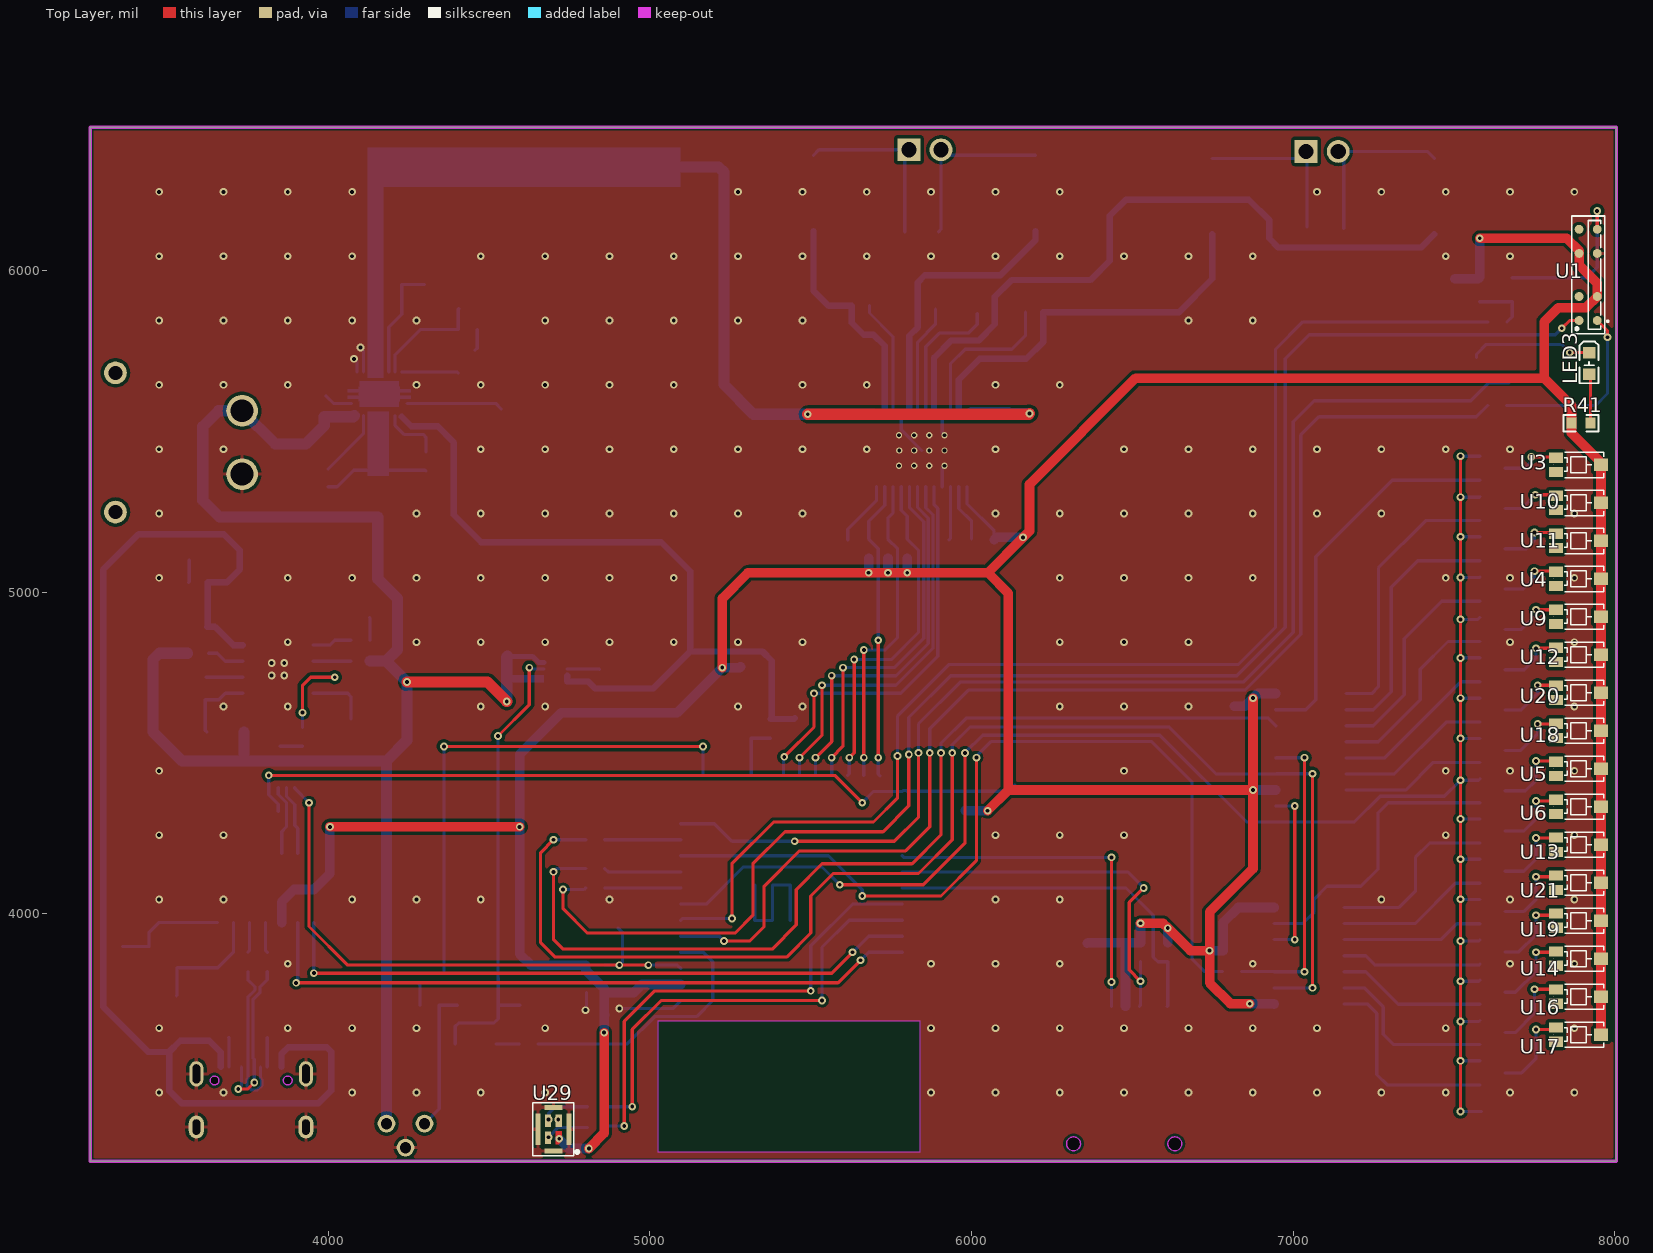
[diagram p0: Top Layer view]
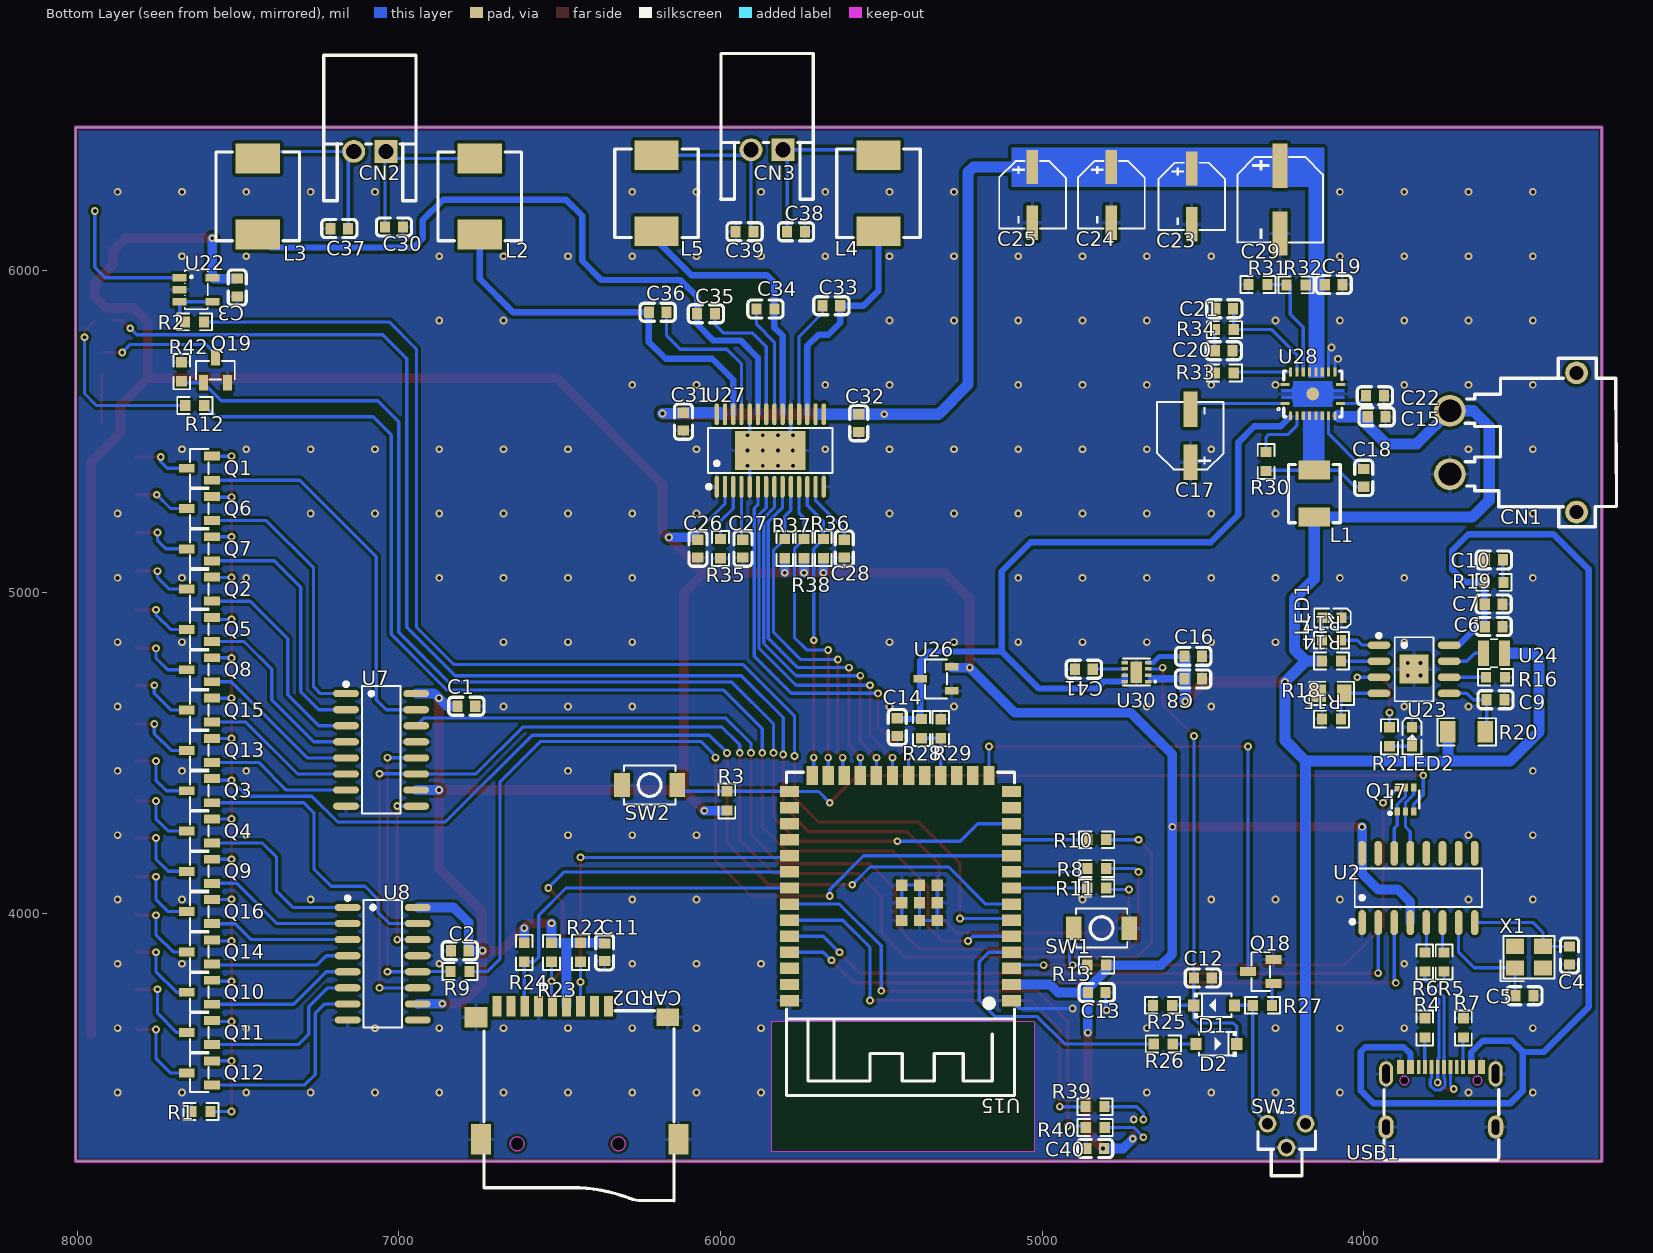
[diagram p1: Bottom Layer view, seen from below]
# Altium PCB MISC75432.pcbdoc (part 1 of 2)
Units mil, origin at the board's own origin, x right, y up, seen from the top; angles counter-clockwise.
Board outline 4745 x 3215 mil, 2 copper layers (Top Layer, Bottom Layer), stack 62.206 mil thick; 150 components, 141 nets, 533 pads, 333 vias.

## Layer stack, top to bottom
Top Solder Mask Layer: solder mask 0.394, Dk 3.3
Top Layer: signal copper 1.379
Dielectric1: surface 59.449, FR4, Dk 4.5
Bottom Layer: signal copper 1.378
Bottom Solder Mask Layer: solder mask 0.394, Dk 3.3

## Board outline
3260,6445 3260,3230 8005,3230 8005,6445

## Design rules (kind name [scope] priority, off if disabled: settings)
BoardOutlineClearance copperThickness2oz_1 [All] p2: genericclearance=7.99 ignorepadtopadclearanceinfootprint=FALSE except(0: Arc-SplitContinuation Track-SplitContinuation SMDPad-SplitContinuation THPad-SplitContinuation Via-SplitContinuation Fill-SplitContinuation Region-SplitContinuation Poly-SplitContinuation Text-SplitContinuation Hole-SplitContinuation; 5.98: Arc-CutoutEdge SMDPad-CutoutEdge THPad-CutoutEdge Via-CutoutEdge Fill-CutoutEdge Region-CutoutEdge Text-CutoutEdge; 6.93: Hole-OutlineEdge Hole-CutoutEdge; 10: Poly-OutlineEdge Poly-CutoutEdge; 11.81: Arc-OutlineEdge Track-OutlineEdge SMDPad-OutlineEdge THPad-OutlineEdge Via-OutlineEdge Fill-OutlineEdge Region-OutlineEdge Text-OutlineEdge Track-CutoutEdge)
BoardOutlineClearance copperThickness1oz_1 [All] p4: genericclearance=4.02 ignorepadtopadclearanceinfootprint=FALSE except(0: Arc-SplitContinuation Track-SplitContinuation SMDPad-SplitContinuation THPad-SplitContinuation Via-SplitContinuation Fill-SplitContinuation Region-SplitContinuation Poly-SplitContinuation Text-SplitContinuation Hole-SplitContinuation; 5.98: SMDPad-CutoutEdge THPad-CutoutEdge Via-CutoutEdge Fill-CutoutEdge Region-CutoutEdge Text-CutoutEdge; 6.93: Hole-OutlineEdge Hole-CutoutEdge; 10: Poly-OutlineEdge Poly-CutoutEdge; 11.81: Arc-OutlineEdge Track-OutlineEdge SMDPad-OutlineEdge THPad-OutlineEdge Via-OutlineEdge Fill-OutlineEdge Region-OutlineEdge Text-OutlineEdge Arc-CutoutEdge Track-CutoutEdge)
Clearance copperThickness2oz [(InNet('OUT_A-') OR InNet('OUT_A+') OR InNet('OUT_B-') OR InNet('OUT_B+'))] p1: gap=7.99 ignorepadtopadclearanceinfootprint=FALSE except(5.98: SMDPad-Track SMDPad-SMDPad THPad-Track SMDPad-THPad THPad-THPad Track-Via SMDPad-Via THPad-Via Via-Via Fill-Track Region-Track Fill-SMDPad Region-SMDPad Fill-THPad Region-THPad Fill-Via Region-Via Fill-Fill Fill-Region Region-Region Arc-Track Arc-SMDPad Arc-THPad Arc-Via Fill-Arc Region-Arc Arc-Arc Text-Track SMDPad-Text Text-THPad Text-Via Fill-Text Region-Text Arc-Text Text-Text; 6.93: Hole-Track Hole-SMDPad Hole-THPad Hole-Via Fill-Hole Region-Hole Hole-Arc Hole-Text; 10: Poly-Track Poly-SMDPad Poly-THPad Poly-Via Poly-Fill Poly-Region Poly-Poly Poly-Arc Poly-Text Poly-Hole)
Clearance copperThickness1oz [All] p3: gap=4.02 ignorepadtopadclearanceinfootprint=FALSE except(5.98: SMDPad-Track SMDPad-SMDPad THPad-Track SMDPad-THPad THPad-THPad Track-Via SMDPad-Via THPad-Via Via-Via Fill-Track Region-Track Fill-SMDPad Region-SMDPad Fill-THPad Region-THPad Fill-Via Region-Via Fill-Fill Fill-Region Region-Region Arc-Track Arc-SMDPad Arc-THPad Arc-Via Fill-Arc Region-Arc Arc-Arc Text-Track SMDPad-Text Text-THPad Text-Via Fill-Text Region-Text Arc-Text Text-Text; 6.93: Hole-Track Hole-SMDPad Hole-THPad Hole-Via Fill-Hole Region-Hole Hole-Arc Hole-Text; 10: Poly-Track Poly-SMDPad Poly-THPad Poly-Via Poly-Fill Poly-Region Poly-Poly Poly-Arc Poly-Text Poly-Hole)
DiffPairsRouting differentialPair [All] p1: maxlimit=6 minlimit=6 mostfreqgap=6 toplayer_minwidth=5 toplayer_prefwidth=10 toplayer_maxwidth=100 toplayer_mingap=6 toplayer_prefgap=6 toplayer_maxgap=6 bottomlayer_minwidth=5 bottomlayer_prefwidth=10 bottomlayer_maxwidth=100 bottomlayer_mingap=6 bottomlayer_prefgap=6 bottomlayer_maxgap=6 maxuncoupledlength=10
HoleToHoleClearance otherClearance [All] p1: gap=11.81 allowstackedmicrovias=TRUE
Length netLength [All] p1: minlimit=0 maxlimit=0
MatchedLengths netLengthTolerance [All] p1: tolerance=1000
PasteMaskExpansion pasteMaskExpansion [All] p1: expansion=0
PlaneConnect innerPlane [All] p1: planeconnectstyle=Relief reliefexpansion=20 reliefentries=4 reliefconductorwidth=10 reliefairgap=10
PolygonConnect copperRegion [(InNet('PD_GATE_15') OR InNet('IO0'))] p1: connectstyle=Relief reliefconductorwidth=10 reliefentries=4 polygonreliefangle="90 Angle" airgapwidth=10 via.connectstyle=Relief via.reliefconductorwidth=10 via.reliefentries=4 via.polygonreliefangle="90 Angle" via.airgapwidth=10
RoutingVias viaSize [All] p1: holewidth=12.01 width=24.02 viastyle="Through Hole" minholewidth=11.81 minwidth=19.68 maxholewidth=248.03 maxwidth=393.7
SolderMaskExpansion solderMaskExpansion [IsVia] p1: expansion=-1000 istentingtop=TRUE
SolderMaskExpansion solderMaskExpansion [All] p2: expansion=2 istentingtop=FALSE
Width copperThickness1oz_2 [All] p1 off: maxlimit=10 minlimit=10 preferedwidth=10 toplayer_minwidth=5 toplayer_maxwidth=100 toplayer_prefwidth=10 bottomlayer_minwidth=5 bottomlayer_maxwidth=100 bottomlayer_prefwidth=10
Width power_trackWidth1 [All] p2 off: maxlimit=10 minlimit=10 preferedwidth=10 toplayer_minwidth=23.6 toplayer_maxwidth=78.7 toplayer_prefwidth=39.4 bottomlayer_minwidth=23.6 bottomlayer_maxwidth=78.7 bottomlayer_prefwidth=39.4
Width trackWidth2 [(InNet('+12V') OR InNet('OUT_A-') OR InNet('OUT_A+') OR InNet('OUT_B-') OR InNet('OUT_B+') OR InNet('VBUS') OR InNet('VSYS_MAIN'))] p3: maxlimit=10 minlimit=10 preferedwidth=10 toplayer_minwidth=15.7 toplayer_maxwidth=39.4 toplayer_prefwidth=19.7 bottomlayer_minwidth=15.7 bottomlayer_maxwidth=39.4 bottomlayer_prefwidth=19.7
Width trackWidth3_BAT [(InNet('VBAT'))] p4: maxlimit=10 minlimit=10 preferedwidth=10 toplayer_minwidth=15.7 toplayer_maxwidth=100 toplayer_prefwidth=59.1 bottomlayer_minwidth=15.7 bottomlayer_maxwidth=100 bottomlayer_prefwidth=59.1
Width copperThickness2oz_2 [All] p5: maxlimit=10 minlimit=10 preferedwidth=10 toplayer_minwidth=8 toplayer_maxwidth=100 toplayer_prefwidth=10 bottomlayer_minwidth=8 bottomlayer_maxwidth=100 bottomlayer_prefwidth=10

## Components (designator, comment, footprint, x,y, rotation, side; value= is the part's Value field where it differs from the comment)
C1 "100nF" C0603 6790,4645 r180 bottom
C2 "100nF" C0603 6810,3885 r0 bottom
C3 "100nF" C0603 7502.44,5946.77 r270 bottom
C4 "22pF" C0603 3360,3870 r90 bottom
C5 "22pF" C0603 3500.12,3745 r0 bottom
C6 "10uF" C0603 3596.03,4892.5 r180 bottom
C7 "22uF" C0603 3596.03,4962.5 r180 bottom
C8 "22uF" C0603 4530,4730 r0 bottom
C9 "22uF" C0603 3590.12,4665 r0 bottom
C10 "10uF" C0603 3595,5100 r0 bottom
C11 "100nF" C0603 6360,3880 r90 bottom
C12 "100nF" C0603 4500,3800 r180 bottom
C13 "1uF" C0603 4830,3755 r0 bottom
C14 "1uF" C0603 5450,4580 r90 bottom
C15 "10uF" C0603 3960,5545 r180 bottom
C16 "100nF" C0603 4529.88,4800 r180 bottom
C17 "2.2uF" CAP-SMD_BD5.0-L5.3-W5.3-LS6.0-FD 4538.41,5485.99 r90 bottom
C18 "100nF" C0603 4000,5355 r270 bottom
C19 "1uF" C0603 4093.41,5955.99 r180 bottom
C20 "22uF" C0603 4435,5750 r180 bottom
C21 "33pF" C0603 4433.41,5880.99 r0 bottom
C22 "47nF" C0603 3965,5610 r180 bottom
C23 "22uF" CAP-SMD_BD5.0-L5.3-W5.3-LS6.3-FD-1 4535,6230 r270 bottom
C24 "22uF" CAP-SMD_BD5.0-L5.3-W5.3-LS6.3-FD-1 4785,6235 r270 bottom
C25 "22uF" CAP-SMD_BD5.0-L5.3-W5.3-LS6.3-FD-1 5030,6235 r270 bottom
C26 "100nF" C0603 6070,5135 r270 bottom
C27 "1uF" C0603 5930,5135 r270 bottom
C28 "1uF" C0603 5615,5135 r90 bottom
C29 "220uF" CAP-SMD_BD6.3-L6.6-W6.6-LS7.3-FD-H7.7 4260,6220 r270 bottom
C30 "680nF" C0603 7015,6135 r180 bottom
C31 "10uF" C0603 6115,5530 r90 bottom
C32 "100nF" C0603 5570,5525 r90 bottom
C33 "220nF" C0603 5655,5890 r180 bottom
C34 "220nF" C0603 5860,5880 r180 bottom
C35 "220nF" C0603 6045,5865 r0 bottom
C36 "220nF" C0603 6195,5870 r0 bottom
C37 "680nF" C0603 7185,6130 r180 bottom
C38 "680nF" C0603 5765,6120 r180 bottom
C39 "680nF" C0603 5925,6120 r180 bottom
C40 "100nF" C0603 4834.88,3270 r0 bottom
C41 "1nF" C0603 4870,4760 r0 bottom
CARD2 "TF-15x15" TF-SMD_TF-15-15 6445,3505 r270 bottom
CN1 "XT30PW-M30.G.Y" CONN-TH_XT30PW-M 3535,5465 r90 bottom
CN2 "S2B-XH-A-1(LF)(SN)" CONN-TH_S2B-XH-A-1-LF-SN 7090,6370 r180 bottom
CN3 "S2B-XH-A-1(LF)(SN)" CONN-TH_S2B-XH-A-1-LF-SN 5855,6375 r180 bottom
D1 "1N4148W" SOD-123_L2.7-W1.6-LS3.7-FD 4465,3715 r0 bottom
D2 "1N4148W" SOD-123_L2.7-W1.6-LS3.7-FD 4458.18,3595.01 r180 bottom
L1 "2.2uH" IND-SMD_L4.6-W4.1_MHCI04015 4153.41,5305.99 r270 bottom
L2 "10uH" IND-SMD_L7.3-W6.8 6748.6,6230 r90 bottom
L3 "10uH" IND-SMD_L7.3-W6.8 7438.6,6230 r90 bottom
L4 "10uH" IND-SMD_L7.3-W6.8 5508.6,6240 r90 bottom
L5 "10uH" IND-SMD_L7.3-W6.8 6198.6,6240 r90 bottom
LED1 "NCD0603Y2" LED0603-RD 4098.98,4919.99 r0 bottom
LED2 "NCD0603Y2" LED0603-RD 3850,4550 r270 bottom
LED3 "GL0603UR01" LED0603-FD 7920,5710 r90 top
Q1 "2N7002" SOT-23-3_L2.9-W1.3-P1.90-LS2.4-BR 7620,5385 r180 bottom
Q2 "2N7002" SOT-23-3_L2.9-W1.3-P1.90-LS2.4-BR 7620,5009 r180 bottom
Q3 "2N7002" SOT-23-3_L2.9-W1.3-P1.90-LS2.4-BR 7620,4382.33 r180 bottom
Q4 "2N7002" SOT-23-3_L2.9-W1.3-P1.90-LS2.4-BR 7620,4257 r180 bottom
Q5 "2N7002" SOT-23-3_L2.9-W1.3-P1.90-LS2.4-BR 7620,4883.67 r180 bottom
Q6 "2N7002" SOT-23-3_L2.9-W1.3-P1.90-LS2.4-BR 7620,5259.67 r180 bottom
Q7 "2N7002" SOT-23-3_L2.9-W1.3-P1.90-LS2.4-BR 7620,5134.33 r180 bottom
Q8 "2N7002" SOT-23-3_L2.9-W1.3-P1.90-LS2.4-BR 7620,4758.33 r180 bottom
Q9 "2N7002" SOT-23-3_L2.9-W1.3-P1.90-LS2.4-BR 7620,4131.67 r180 bottom
Q10 "2N7002" SOT-23-3_L2.9-W1.3-P1.90-LS2.4-BR 7620,3755.67 r180 bottom
Q11 "2N7002" SOT-23-3_L2.9-W1.3-P1.90-LS2.4-BR 7620,3630.33 r180 bottom
Q12 "2N7002" SOT-23-3_L2.9-W1.3-P1.90-LS2.4-BR 7620,3505 r180 bottom
Q13 "2N7002" SOT-23-3_L2.9-W1.3-P1.90-LS2.4-BR 7620,4507.67 r180 bottom
Q14 "2N7002" SOT-23-3_L2.9-W1.3-P1.90-LS2.4-BR 7620,3881 r180 bottom
Q15 "2N7002" SOT-23-3_L2.9-W1.3-P1.90-LS2.4-BR 7620,4633 r180 bottom
Q16 "2N7002" SOT-23-3_L2.9-W1.3-P1.90-LS2.4-BR 7620,4006.33 r180 bottom
Q17 "UMH3N" SC-70-6_L2.2-W1.3-P0.65-LS2.1-BR 3870,4355 r270 bottom
Q18 "2N7002" SOT-23-3_L2.9-W1.3-P1.90-LS2.4-BR 4320,3820 r180 bottom
Q19 "2N7002" SOT-23-3_L2.9-W1.3-P1.90-LS2.4-BR 7570,5690 r270 bottom
R1 "10kΩ" R0603 7615,3385 r0 bottom
R2 "49.9Ω" R0603 7635,5840 r180 bottom
R3 "10kΩ" R0603 5980,4350.68 r270 bottom
R4 "5.1kΩ" R0603 3810,3645 r270 bottom
R5 "27Ω" R0603 3750,3850 r270 bottom
R6 "27Ω" R0603 3810,3850 r270 bottom
R7 "5.1kΩ" R0603 3690,3645 r270 bottom
R8 "49.9Ω" R0603 4830,4140 r180 bottom
R9 "49.9Ω" R0603 6810,3820 r0 bottom
R10 "49.9Ω" R0603 4830,4230 r0 bottom
R11 "49.9Ω" R0603 4830,4080 r0 bottom
R12 "49.9Ω" R0603 7634.32,5580 r180 bottom
R13 "10kΩ" R0603 4830,3840 r0 bottom
R14 "1kΩ" R0603 4100,4785.34 r180 bottom
R15 "82kΩ" R0603 4100,4605 r180 bottom
R16 "47kΩ" R0603 3590,4735 r180 bottom
R17 "100Ω" R0603 4100,4850 r180 bottom
R18 "HNTC0805-104F3950FB" R0805 4100,4685 r180 bottom
R19 "2Ω" R0603 3595,5030 r180 bottom
R20 "500mΩ" R1206 3680,4565 r0 bottom
R21 "100Ω" R0603 3920,4550 r90 bottom
R22 "4.7kΩ" R0603 6435,3880 r270 bottom
R23 "4.7kΩ" R0603 6525,3880 r270 bottom
R24 "4.7kΩ" R0603 6610,3880 r270 bottom
R25 "1MΩ" R0603 4625,3715 r0 bottom
R26 "10kΩ" R0603 4623.18,3595.01 r180 bottom
R27 "100kΩ" R0603 4315,3715 r0 bottom
R28 "499kΩ" R0603 5374.66,4575.34 r90 bottom
R29 "100kΩ" R0603 5315,4575 r270 bottom
R30 "249kΩ" R0603 4303.41,5405.99 r270 bottom
R31 "20kΩ" R0603 4328.41,5955.99 r180 bottom
R32 "180kΩ" R0603 4210,5955 r180 bottom
R33 "100kΩ" R0603 4433.41,5680.99 r180 bottom
R34 "10kΩ" R0603 4433.41,5815.99 r0 bottom
R35 "4.7kΩ" R0603 6000,5135 r90 bottom
R36 "10kΩ" R0603 5680,5135 r90 bottom
R37 "2.2kΩ" R0603 5800,5135 r90 bottom
R38 "2.2kΩ" R0603 5740,5135 r90 bottom
R39 "33Ω" R0603 4835.68,3400 r180 bottom
R40 "33Ω" R0603 4834.66,3335.34 r180 bottom
R41 "56Ω" R0603 7895,5525 r0 top
R42 "10kΩ" R0603 7675,5685 r90 bottom
SW1 "TS-1088-AR02016" SW-SMD_L3.9-W3.0-P4.45 4815,3955 r0 bottom
SW2 "TS-1088-AR02016" SW-SMD_L3.9-W3.0-P4.45 6220,4400 r0 bottom
SW3 "TS-1009B-05026" SW-TH_3P-L4.5-W3.8-P3.10-LS1.9_TS-1009B-05026 4240,3310 r180 bottom
U1 "S13131-1536" BGA-8_L9.1-W2.4_S13131-1536 7917.16,5985.9 r90 top
U2 "CH340G" SOIC-16_L9.9-W3.9-P1.27-LS6.0-BL 3830,4080 r180 bottom
U3 "TEMT6000X01" SENSORS-SMD_TEMT6000X01 7886.89,5395.35 r0 top
U4 "TEMT6000X01" SENSORS-SMD_TEMT6000X01 7886.89,5041.02 r0 top
U5 "TEMT6000X01" SENSORS-SMD_TEMT6000X01 7886.89,4450.47 r0 top
U6 "TEMT6000X01" SENSORS-SMD_TEMT6000X01 7886.89,4332.36 r0 top
U7 "74HC595" SOP-16_L9.9-W3.9-P1.27-LS6.0-BL 7055,4509.33 r270 bottom
U8 "74HC595" SOP-16_L9.9-W3.9-P1.27-LS6.0-BL 7050,3844.33 r270 bottom
U9 "TEMT6000X01" SENSORS-SMD_TEMT6000X01 7886.89,4922.91 r0 top
U10 "TEMT6000X01" SENSORS-SMD_TEMT6000X01 7886.89,5277.24 r0 top
U11 "TEMT6000X01" SENSORS-SMD_TEMT6000X01 7886.89,5159.13 r0 top
U12 "TEMT6000X01" SENSORS-SMD_TEMT6000X01 7886.89,4804.8 r0 top
U13 "TEMT6000X01" SENSORS-SMD_TEMT6000X01 7886.89,4214.25 r0 top
U14 "TEMT6000X01" SENSORS-SMD_TEMT6000X01 7886.89,3859.92 r0 top
U15 "ESP32-S3-WROOM-1-N8R8" WIRELM-SMD_ESP32-S3-WROOM-1 5440,4080 r0 bottom
U16 "TEMT6000X01" SENSORS-SMD_TEMT6000X01 7886.89,3741.81 r0 top
U17 "TEMT6000X01" SENSORS-SMD_TEMT6000X01 7886.89,3623.7 r0 top
U18 "TEMT6000X01" SENSORS-SMD_TEMT6000X01 7886.89,4568.58 r0 top
U19 "TEMT6000X01" SENSORS-SMD_TEMT6000X01 7886.89,3978.03 r0 top
U20 "TEMT6000X01" SENSORS-SMD_TEMT6000X01 7886.89,4686.69 r0 top
U21 "TEMT6000X01" SENSORS-SMD_TEMT6000X01 7886.89,4096.14 r0 top
U22 "LMV321IDBVR" SOT-23-5_L3.0-W1.7-P0.95-LS2.8-BR 7630,5940 r0 bottom
U23 "IP2312U_VSET" SOP-8_L4.9-W3.9-P1.27-LS6.0-BL-EP 3843.52,4760 r270 bottom
U24 "1uH" IND-SMD_L2.5-W2.0-VLS252012CX-150M 3595,4810 r180 bottom
U26 "ME6211A33M3G-N" SOT-23-3_L2.9-W1.6-P1.90-LS2.8-BR 5330,4730 r180 bottom
U27 "TAS5805MPWPR" HTSSOP-28_L9.7-W4.4-P0.65-LS6.4-BL-EP 5845,5440 r180 bottom
U28 "TPS61088RHLR" VQFN-20_L4.6-W3.6-P0.50-BL 4158.41,5615.99 r180 bottom
U29 "MSM261DHP006" QFN-8_L4.0-W3.0_WMM7040DTHN0-8-TR 4700,3330 r0 top
U30 "TPS22965DSGR" UDFN-8_L2.0-W2.0-P0.50-TL-EP 4706.58,4751.21 r0 bottom
USB1 "TYPE-C 16PIN 2MD(073)" USB-C-SMD_TYPE-C-6PIN-2MD-073 3760,3430 r180 bottom
X1 "12MHz" CRYSTAL-SMD_4P-L3.2-W2.5-BL 3486.01,3864.99 r180 bottom

## Footprints (in the part's own frame and the unit in brackets; to place one, negate y for a bottom-side part, rotate by r counter-clockwise, add the part's x,y. Pads: shape width x height; smd on the part's side, far side on the other; paste and mask are expansions set on the pad)
BGA-8_L9.1-W2.4_S13131-1536 [mm]
  round 0.7 smd paste+0 mask+0.05: 1(-3.6,-0.72) 2(-1.7,-0.72) 3(1.7,-0.72) 4(3.6,-0.72) 5(3.6,0.72) 6(1.7,0.72) 7(-1.7,0.72) 8(-3.6,0.72)
  silkscreen extent -4.65,-1.62 4.65,1.3
C0603 [mm]
  rect 0.8x0.9 smd: 1(-0.7,0) 2(0.7,0)
  silkscreen extent -1.39,-0.71 1.39,0.71
CAP-SMD_BD5.0-L5.3-W5.3-LS6.0-FD [mm]
  rect 2.8x1.1 smd: 1(-2.1,0) 2(2.1,0)
  silkscreen extent -2.66,-2.62 2.66,2.65
CAP-SMD_BD5.0-L5.3-W5.3-LS6.3-FD-1 [mm]
  rect 2.7x0.91 smd: 1(-2.2,0) 2(2.2,0)
  silkscreen extent -2.66,-2.62 2.66,2.65
CAP-SMD_BD6.3-L6.6-W6.6-LS7.3-FD-H7.7 [mm]
  rect 3.5x1.2 smd: 1(-2.67,0) 2(2.67,0)
  silkscreen extent -3.38,-3.38 3.38,3.38
CONN-TH_S2B-XH-A-1-LF-SN [mm]
  rect 1.8x1.8 hole 1.2: 1(1.27,0)
  round 1.8 hole 1.2: 2(-1.27,0)
  silkscreen extent -3.65,-3.9 3.64,7.6
CONN-TH_XT30PW-M [mm]
  round 2.5 hole 1.8: 1(-2.5,5) 2(2.5,5)
  round 1.8 hole 1.1: 3(5.5,-5) 4(-5.5,-5)
  silkscreen extent -6.65,-8.15 6.65,3.81
CRYSTAL-SMD_4P-L3.2-W2.5-BL [mm]
  rect 1.4x1.2 smd: 1(-1.1,-0.85) 2(1.1,-0.85) 3(1.1,0.85) 4(-1.1,0.85)
  silkscreen extent -2.26,-1.91 2.03,1.68
HTSSOP-28_L9.7-W4.4-P0.65-LS6.4-BL-EP [mm]
  oval 0.343x1.731 smd: 1(-4.225,-2.866) 2(-3.575,-2.866) 3(-2.925,-2.866) 4(-2.275,-2.866) 5(-1.625,-2.866) 6(-0.975,-2.866) 7(-0.325,-2.866) 8(0.325,-2.866) 9(0.975,-2.866) 10(1.625,-2.866) 11(2.275,-2.866) 12(2.925,-2.866) 13(3.575,-2.866) 14(4.225,-2.866) 15(4.225,2.866) 16(3.575,2.866) 17(2.925,2.866) 18(2.275,2.866) 19(1.625,2.866) 20(0.975,2.866) 21(0.325,2.866) 22(-0.325,2.866) 23(-0.975,2.866) 24(-1.625,2.866) 25(-2.275,2.866) 26(-2.925,2.866) 27(-3.575,2.866) 28(-4.225,2.866)
  rect 5.6x3.1 smd paste+0 mask+0.05: 29(0,0)
  silkscreen extent -5,-3.02 4.93,1.77
IND-SMD_L2.5-W2.0-VLS252012CX-150M [mm]
  rect 0.85x2 smd: 1(-0.83,0) 2(0.83,0)
  silkscreen extent -0.29,-1.1 0.29,1.1
IND-SMD_L4.6-W4.1_MHCI04015 [mm]
  rect 1.5x2.5 smd: 1(-1.85,0) 2(1.85,0)
  silkscreen extent -2.3,-2.05 2.3,2.05
IND-SMD_L7.3-W6.8 [mm]
  rect 2.35x3.5 smd: 1(-3,0) 2(3,0)
  silkscreen extent -3.5,-3.3 3.5,3.3
LED0603-FD [mm]
  rect 0.9x1 smd: 1(-0.85,0) 2(0.85,0)
  silkscreen extent -1.55,-0.75 1.75,0.75
LED0603-RD [mm]
  rect 0.8x0.8 smd: 1(-0.749,0) 2(0.749,0)
  silkscreen extent -1.49,-0.75 1.39,0.76
QFN-8_L4.0-W3.0_WMM7040DTHN0-8-TR [mm]
  round 0.239 smd: 1(0.414,-0.647)
  rect 0.5x1 smd paste+0 mask+0.05: 2(0.425,0.675) 3(-0.425,0.675) 4(-0.425,-0.675)
  rect 1.4x0.4 smd paste+0 mask+0.05: 5(0,-1.725) 7(0,1.725)
  rect 0.4x2.5 smd paste+0 mask+0.05: 6(1.225,0) 8(-1.225,0)
  Top Layer region: 0.175,-0.175 0.675,-0.175 0.675,-0.925 0.425,-1.175 0.175,-1.175
  silkscreen extent -1.62,-2.09 1.99,2.1
R0603 [mil]
  rect 31.75x34.02 smd paste-3937.01 mask+2: 1(-29.66,0) 2(29.66,0)
  silkscreen extent -55,-26 55,26
R0805 [mm]
  rect 1.133x1.377 smd paste-100 mask+0.051: 1(-1,0) 2(1,0)
  silkscreen extent -1.76,-0.92 1.76,0.92
R1206 [mil]
  rect 47.54x66.97 smd paste-3937.01 mask+2: 1(-58.22,0) 2(58.22,0)
  silkscreen extent -91,-42 91,42
SC-70-6_L2.2-W1.3-P0.65-LS2.1-BR [mm]
  rect 0.6x0.42 smd: 1(0.95,-0.65) 2(0.95,0) 3(0.95,0.65) 4(-0.95,0.65) 5(-0.95,0) 6(-0.95,-0.65)
  silkscreen extent -0.7,-1.34 1.22,1.1
SENSORS-SMD_TEMT6000X01 [mil]
  rect 43.3x31.5 smd: 1(-70,22) 2(-70,-22)
  rect 43.3x39.4 smd: 3(70,0)
  silkscreen extent -79,-39 79,39
SOD-123_L2.7-W1.6-LS3.7-FD [mm]
  rect 0.88x0.96 smd: 1(-1.61,0) 2(1.61,0)
  silkscreen extent -1.38,-1 1.6,1
SOIC-16_L9.9-W3.9-P1.27-LS6.0-BL [mil]
  oval 23.7x77.6 smd: 1(-175,-107.7) 2(-125,-107.7) 3(-75,-107.7) 4(-25,-107.7) 5(25,-107.7) 6(75,-107.7) 7(125,-107.7) 8(175,-107.7) 9(175,107.7) 10(125,107.7) 11(75,107.7) 12(25,107.7) 13(-25,107.7) 14(-75,107.7) 15(-125,107.7) 16(-175,107.7)
  silkscreen extent -211,-111 198,60
SOP-8_L4.9-W3.9-P1.27-LS6.0-BL-EP [mm]
  oval 0.6x1.8 smd: 1(-1.905,-2.772) 2(-0.635,-2.772) 3(0.635,-2.772) 4(1.905,-2.772) 5(1.905,2.772) 6(0.635,2.772) 7(-0.635,2.772) 8(-1.905,2.772)
  rect 2.29x2.29 smd: 9(0,0)
  silkscreen extent -2.8,-2.92 2.53,1.52
SOP-16_L9.9-W3.9-P1.27-LS6.0-BL [mil]
  oval 22.6x80.24 smd: 1(-175,-109.02) 2(-125,-109.02) 3(-75,-109.02) 4(-25,-109.02) 5(25,-109.02) 6(75,-109.02) 7(125,-109.02) 8(175,-109.02) 9(175,109.02) 10(125,109.02) 11(75,109.02) 12(25,109.02) 13(-25,109.02) 14(-75,109.02) 15(-125,109.02) 16(-175,109.02)
  silkscreen extent -210,-115 198,60
SOT-23-3_L2.9-W1.3-P1.90-LS2.4-BR [mm]
  rect 1.25x0.7 smd: 1(1,-0.95) 2(1,0.95) 3(-1,0)
  silkscreen extent -0.73,-1.53 0.73,1.53
SOT-23-3_L2.9-W1.6-P1.90-LS2.8-BR [mm]
  rect 1.07x0.6 smd: 1(1.235,-0.95) 2(1.235,0.95) 3(-1.235,0)
  silkscreen extent -0.88,-1.54 0.88,1.54
SOT-23-5_L3.0-W1.7-P0.95-LS2.8-BR [mm]
  rect 1.1x0.6 smd: 1(1.3,-0.95) 2(1.3,0) 3(1.3,0.95) 4(-1.3,0.95) 5(-1.3,-0.95)
  silkscreen extent -0.9,-1.55 0.9,1.55
SW-SMD_L3.9-W3.0-P4.45 [mm]
  rect 1.23x1.86 smd: 1(-2.185,0) 2(2.185,0)
  silkscreen extent -2.03,-1.54 2.03,1.54
SW-TH_3P-L4.5-W3.8-P3.10-LS1.9_TS-1009B-05026 [mm]
  round 1.4 hole 0.9: 1(1.5,0.95) 2(-1.5,0.95) 3(0,-0.95)
  silkscreen extent -2.25,-3.18 2.3,1.83
TF-SMD_TF-15-15 [mil]
  rect 63x27.6 smd: 1(-206.75,96.45) 2(-206.75,53.15) 3(-206.75,9.84) 4(-206.75,-33.47) 5(-206.75,-76.77) 6(-206.75,-120.08) 7(-206.75,-163.39) 8(-206.75,-206.7) 9(-206.75,-250)
  rect 63x70.87 smd: 10(-173.17,-314.96)
  rect 94.49x62.99 smd: 11(206.75,-299.22) 12(206.75,314.96)
  rect 55.1x70.9 smd: 13(-173.15,281.51)
  Board Outline Layer circle w0.1: c220.53,-187.01 r21.65
  Board Outline Layer circle w0.1: c220.53,127.95 r21.65
  Board Outline Layer region: 220.53,-208.66 229.93,-206.52 237.46,-200.51 241.64,-191.83 241.64,-182.19 237.46,-173.51 229.93,-167.5 220.53,-165.36 220.53,-165.36 211.13,-167.5 203.6,-173.51 199.42,-182.19 199.42,-191.83 203.6,-200.51 211.13,-206.52 220.53,-208.66
  Board Outline Layer region: 220.53,-208.66 224.51,-208.3 228.35,-207.2 231.93,-205.42 235.12,-203.01 237.81,-200.06 239.91,-196.66 241.36,-192.94 242.09,-189.01 242.09,-185.01 241.36,-181.08 239.91,-177.36 237.81,-173.96 235.12,-171.01 231.93,-168.6 228.35,-166.82 224.51,-165.72 220.53,-165.36 216.55,-165.72 212.71,-166.82 209.13,-168.6 205.94,-171.01 203.25,-173.96 201.15,-177.36 199.7,-181.08 198.97,-185.01 198.97,-189.01 199.7,-192.94 201.15,-196.66 203.25,-200.06 205.94,-203.01 209.13,-205.42 212.71,-207.2 216.55,-208.3
  Board Outline Layer region: 220.53,106.3 229.93,108.44 237.46,114.45 241.64,123.13 241.64,132.77 237.46,141.45 229.93,147.46 220.53,149.6 220.53,149.6 211.13,147.46 203.6,141.45 199.42,132.77 199.42,123.13 203.6,114.45 211.13,108.44 220.53,106.3
  Board Outline Layer region: 220.53,106.3 224.51,106.66 228.35,107.76 231.93,109.54 235.12,111.95 237.81,114.9 239.91,118.3 241.36,122.02 242.09,125.95 242.09,129.95 241.36,133.88 239.91,137.6 237.81,141 235.12,143.95 231.93,146.36 228.35,148.14 224.51,149.24 220.53,149.6 216.55,149.24 212.71,148.14 209.13,146.36 205.94,143.95 203.25,141 201.15,137.6 199.7,133.88 198.97,129.95 198.97,125.95 199.7,122.02 201.15,118.3 203.25,114.9 205.94,111.95 209.13,109.54 212.71,107.76 216.55,106.66
  Multi-Layer board cut-out: 220.53,-208.66 229.93,-206.52 237.46,-200.51 241.64,-191.83 241.64,-182.19 237.46,-173.51 229.93,-167.5 220.53,-165.36 220.53,-165.36 211.13,-167.5 203.6,-173.51 199.42,-182.19 199.42,-191.83 203.6,-200.51 211.13,-206.52 220.53,-208.66
  Multi-Layer board cut-out: 220.53,106.3 229.93,108.44 237.46,114.45 241.64,123.13 241.64,132.77 237.46,141.45 229.93,147.46 220.53,149.6 220.53,149.6 211.13,147.46 203.6,141.45 199.42,132.77 199.42,123.13 203.6,114.45 211.13,108.44 220.53,106.3
  silkscreen extent -193,-290 398,301
UDFN-8_L2.0-W2.0-P0.50-TL-EP [mm]
  rect 0.505x0.28 smd: 1(-0.928,0.75) 2(-0.928,0.25) 3(-0.928,-0.25) 4(-0.928,-0.75) 5(0.928,-0.75) 6(0.928,-0.25) 7(0.928,0.25) 8(0.928,0.75)
  rect 0.9x1.7 smd: 9(0,0)
  silkscreen extent -1.55,-1.08 1.08,1.08
USB-C-SMD_TYPE-C-6PIN-2MD-073 [mm]
  rect 0.55x1.1 smd paste-100 mask+0.05: 1(-3.2,2.375) 2(-2.4,2.375) 11(2.4,2.375) 12(3.2,2.375)
  rect 0.3x1.1 smd paste-100 mask+0.05: 3(-1.75,2.375) 4(-1.25,2.375) 5(-0.75,2.375) 6(-0.25,2.375) 7(0.25,2.375) 8(0.75,2.375) 9(1.25,2.375) 10(1.75,2.375)
  oval 1.2x1.8 hole 0.6 slot 1.2 at 90 deg paste+0 mask+0.05: 13(-4.325,-2.375) 14(4.325,-2.375)
  oval 1.1x2 hole 0.6 slot 1.5 at 90 deg paste+0 mask+0.05: 13(-4.325,1.825) 14(4.325,1.825)
  Board Outline Layer circle w0.003: c-2.89,1.305 r0.35
  Board Outline Layer circle w0.003: c2.89,1.305 r0.35
  Board Outline Layer region: -3.24,1.305 -3.205,1.153 -3.108,1.031 -2.968,0.964 -2.812,0.964 -2.672,1.031 -2.575,1.153 -2.54,1.305 -2.54,1.305 -2.575,1.457 -2.672,1.579 -2.812,1.646 -2.968,1.646 -3.108,1.579 -3.205,1.457 -3.24,1.305
  Board Outline Layer region: -3.24,1.305 -3.231,1.227 -3.205,1.153 -3.164,1.087 -3.108,1.031 -3.042,0.99 -2.968,0.964 -2.89,0.955 -2.812,0.964 -2.738,0.99 -2.672,1.031 -2.616,1.087 -2.575,1.153 -2.549,1.227 -2.54,1.305 -2.549,1.383 -2.575,1.457 -2.616,1.523 -2.672,1.579 -2.738,1.62 -2.812,1.646 -2.89,1.655 -2.968,1.646 -3.042,1.62 -3.108,1.579 -3.164,1.523 -3.205,1.457 -3.231,1.383
  Board Outline Layer region: 2.54,1.305 2.575,1.153 2.672,1.031 2.812,0.964 2.968,0.964 3.108,1.031 3.205,1.153 3.24,1.305 3.24,1.305 3.205,1.457 3.108,1.579 2.968,1.646 2.812,1.646 2.672,1.579 2.575,1.457 2.54,1.305
  Board Outline Layer region: 2.54,1.305 2.549,1.227 2.575,1.153 2.616,1.087 2.672,1.031 2.738,0.99 2.812,0.964 2.89,0.955 2.968,0.964 3.042,0.99 3.108,1.031 3.164,1.087 3.205,1.153 3.231,1.227 3.24,1.305 3.231,1.383 3.205,1.457 3.164,1.523 3.108,1.579 3.042,1.62 2.968,1.646 2.89,1.655 2.812,1.646 2.738,1.62 2.672,1.579 2.616,1.523 2.575,1.457 2.549,1.383
  Multi-Layer board cut-out: -3.24,1.305 -3.205,1.153 -3.108,1.031 -2.968,0.964 -2.812,0.964 -2.672,1.031 -2.575,1.153 -2.54,1.305 -2.54,1.305 -2.575,1.457 -2.672,1.579 -2.812,1.646 -2.968,1.646 -3.108,1.579 -3.205,1.457 -3.24,1.305
  Multi-Layer board cut-out: 2.54,1.305 2.575,1.153 2.672,1.031 2.812,0.964 2.968,0.964 3.108,1.031 3.205,1.153 3.24,1.305 3.24,1.305 3.205,1.457 3.108,1.579 2.968,1.646 2.812,1.646 2.672,1.579 2.575,1.457 2.54,1.305
  silkscreen extent -4.5,-4.97 4.57,0.6
VQFN-20_L4.6-W3.6-P0.50-BL [mm]
  rect 0.7x0.244 smd paste+0 mask+0.05: 1(-2.185,-0.75) 10(2.185,-0.75) 11(2.185,0.75) 20(-2.185,0.75)
  rect 0.244x0.7 smd paste+0 mask+0.05: 2(-1.748,-1.727) 3(-1.248,-1.727) 4(-0.748,-1.727) 5(-0.248,-1.727) 6(0.252,-1.727) 7(0.752,-1.727) 8(1.252,-1.727) 9(1.752,-1.727) 12(1.752,1.727) 13(1.252,1.727) 14(0.752,1.727) 15(0.252,1.727) 16(-0.248,1.727) 17(-0.748,1.727) 18(-1.248,1.727) 19(-1.748,1.727)
  round 1.015 smd: 21(0.002,0.001)
  Top Layer region: -1.621,0.143 -2.485,0.146 -2.485,0.376 -1.621,0.38 -1.618,0.565 -1.522,0.566 -1.521,1.016 1.526,1.016 1.523,0.571 1.621,0.571 1.624,0.381 2.485,0.381 2.485,0.147 1.621,0.147 1.624,-0.137 2.485,-0.137 2.485,-0.371 1.621,-0.371 1.624,-0.561 1.526,-0.561 1.526,-1.014 -1.522,-1.016 -1.522,-0.567 -1.62,-0.567 -1.619,-0.374 -2.481,-0.374 -2.48,-0.143 -1.618,-0.144 -1.619,0.145
  silkscreen extent -2.8,-1.8 2.3,1.8
WIRELM-SMD_ESP32-S3-WROOM-1 [mm]
  rect 1.5x0.9 smd paste+0 mask+0.05: 1(-8.75,8.895) 2(-8.75,7.625) 3(-8.75,6.355) 4(-8.75,5.085) 5(-8.75,3.815) 6(-8.75,2.545) 7(-8.75,1.275) 8(-8.75,0.005) 9(-8.75,-1.265) 10(-8.75,-2.535) 11(-8.75,-3.805) 12(-8.75,-5.075) 13(-8.75,-6.345) 14(-8.75,-7.615) 27(8.75,-7.615) 28(8.75,-6.345) 29(8.75,-5.075) 30(8.75,-3.805) 31(8.75,-2.535) 32(8.75,-1.265) 33(8.75,0.005) 34(8.75,1.275) 35(8.75,2.545) 36(8.75,3.815) 37(8.75,5.085) 38(8.75,6.355) 39(8.75,7.625) 40(8.75,8.895)
  rect 0.9x1.5 smd paste+0 mask+0.05: 15(-6.985,-8.895) 16(-5.715,-8.895) 17(-4.445,-8.895) 18(-3.175,-8.895) 19(-1.905,-8.895) 20(-0.635,-8.895) 21(0.635,-8.895) 22(1.905,-8.895) 23(3.175,-8.895) 24(4.445,-8.895) 25(5.715,-8.895) 26(6.985,-8.865)
  rect 0.9x0.9 smd: 41(-2.9,-0.225) 41(-2.9,1.175) 41(-2.9,2.575) 41(-1.5,-0.225) 41(-1.5,1.175) 41(-1.5,2.575) 41(-0.1,-0.225) 41(-0.1,1.175) 41(-0.1,2.575)
  silkscreen extent -9,-9.14 9.02,16.39

## Via types
v1: diameter 24.02, hole 12, Top Layer to Bottom Layer, 317 vias
v2: diameter 19.69, hole 11.8, Top Layer to Bottom Layer, 12 vias
v3: diameter 24, hole 12, Top Layer to Bottom Layer, 4 vias

## Nets (pads, with @x,y where several pads share a name; then routed paths per layer and width w, separated by ;. In a path a pad name is that pad's centre, name@x,y a point inside that pad or via, vN(x,y) a via of type N, cw(c..) or ccw(c..) an arc to the next point about the centre after c; other vN are vias at no path point)
$1N31: U8.9
$1N50: U1.7
$1N52: U1.5
$1N74: Q2.3 U4.1 | length 193.3
  Top Layer w10: v1(7750,5065) 7814.91,5065 U4.1@7816.89,5063.02
  Bottom Layer w10: Q2.3@7659.37,5009 7714,5009 7750,5045 v1(7750,5065)
$1N149: R2.1 U22.3 U22.4 | length 171.8
  Bottom Layer w10: U22.4@7578.81,5902.6 U22.3@7681.19,5902.6 7681.19,5856.52 R2.1@7664.66,5840
$1N152: Q1.3 U3.1 | length 181.9
  Top Layer w10: v1(7740,5420) 7814.24,5420 U3.1@7816.89,5417.35
  Bottom Layer w10: Q1.3@7659.37,5385 7720,5385 7740,5405 v1(7740,5420)
$1N154: Q6.3 U10.1 | length 176.6
  Top Layer w10: v1(7752.5,5302.5) 7813.63,5302.5 U10.1@7816.89,5299.24
  Bottom Layer w10: Q6.3@7659.37,5259.67 7709.67,5259.67 v1(7752.5,5302.5)
$1N158: Q5.3 U9.1 | length 191.7
  Top Layer w10: v1(7755,4945) 7816.8,4945 U9.1@7816.89,4944.91
  Bottom Layer w10: Q5.3@7659.37,4883.67 7708.67,4883.67 7755,4930 v1(7755,4945)
$1N159: Q7.3 U11.1 | length 194.8
  Top Layer w10: v1(7750,5185) 7813.02,5185 U11.1@7816.89,5181.13
  Bottom Layer w10: Q7.3@7659.37,5134.33 7724.33,5134.33 7750,5160 v1(7750,5185)
$1N162: Q8.3 U12.1 | length 203.5
  Top Layer w10: v1(7755,4825) 7815.09,4825 U12.1@7816.89,4826.8
  Bottom Layer w10: Q8.3@7659.37,4758.33 7718.33,4758.33 7755,4795 v1(7755,4825)
$1N164: Q3.3 U5.1 | length 232.1
  Top Layer w10: v1(7755,4475) 7814.36,4475 U5.1@7816.89,4472.47
  Bottom Layer w10: Q3.3@7659.37,4382.33 7722.33,4382.33 7755,4415 v1(7755,4475)
$1N166: Q4.3 U6.1 | length 230.1
  Top Layer w10: v1(7755,4350) 7812.53,4350 U6.1@7816.89,4354.36
  Bottom Layer w10: Q4.3@7659.37,4257 7717,4257 7755,4295 v1(7755,4350)
$1N168: Q9.3 U13.1 | length 238.9
  Top Layer w10: v1(7755,4235) 7815.64,4235 U13.1@7816.89,4236.25
  Bottom Layer w10: Q9.3@7659.37,4131.67 7716.67,4131.67 7755,4170 v1(7755,4235)
$1N170: Q13.3 U18.1 | length 209.4
  Top Layer w10: v1(7760,4590) 7816.31,4590 U18.1@7816.89,4590.58
  Bottom Layer w10: Q13.3@7659.37,4507.67 7707.67,4507.67 7760,4560 v1(7760,4590)
$1N173: Q14.3 U19.1 | length 242
  Top Layer w10: v1(7755,3995) 7811.86,3995 U19.1@7816.89,4000.03
  Bottom Layer w10: Q14.3@7659.37,3881 7701,3881 7755,3935 v1(7755,3995)
$1N175: Q15.3 U20.1 | length 204.6
  Top Layer w10: v1(7760,4710) 7815.58,4710 U20.1@7816.89,4708.69
  Bottom Layer w10: Q15.3@7659.37,4633 7708,4633 7760,4685 v1(7760,4710)
$1N177: Q16.3 U21.1 | length 244.8
  Top Layer w10: v1(7755,4115) 7813.75,4115 U21.1@7816.89,4118.14
  Bottom Layer w10: Q16.3@7659.37,4006.33 7716.33,4006.33 7755,4045 v1(7755,4115)
$1N179: Q10.3 U14.1 | length 245
  Top Layer w10: v1(7755,3880) 7814.97,3880 U14.1@7816.89,3881.92
  Bottom Layer w10: Q10.3@7659.37,3755.67 7690.67,3755.67 7755,3820 v1(7755,3880)
$1N181: Q11.3 U16.1 | length 257.7
  Top Layer w10: v1(7750,3765) 7815.7,3765 U16.1@7816.89,3763.81
  Bottom Layer w10: Q11.3@7659.37,3630.33 7690.33,3630.33 7750,3690 v1(7750,3765)
$1N183: Q12.3 U17.1 | length 268.5
  Top Layer w10: v1(7755,3640) 7811.19,3640 U17.1@7816.89,3645.7
  Bottom Layer w10: Q12.3@7659.37,3505 7710,3505 7755,3550 v1(7755,3640)
$1N190: LED3.1 R41.2 | length 153.5
  Top Layer w10: LED3.1@7920,5676.53 7924.66,5671.88 R41.2@7924.66,5525
$1N191: LED3.2 Q19.3 | length 384
  Top Layer w10: v1(7860,5745) 7918.47,5745 LED3.2@7920,5743.47
  Bottom Layer w10: Q19.3@7570,5729.37 7570,5740 7600,5770 7835,5770 v1(7860,5745)
$2N8: U15.19
$2N10: U15.17
$2N11: U15.16
$2N14: U15.28
$2N24: U15.38
$2N25: U15.39
$2N27: U15.14
$2N28: U15.13
$2N36: R12.2 U15.5 | length 3820
  Top Layer w10: v1(5230,3915) 5310,3915 5355,3960 5355,4085 5465,4195 5795,4195 5870,4270 v1(5870,4500)
  Bottom Layer w10: U15.5@5095.51,3929.8 5215.19,3929.8 v1(5230,3915) ; v1(5870,4500) 5870,4575 5990,4695 6850,4695 7023.54,4868.54 7023.54,5488.54 7080,5545 7569.66,5545 R12.2@7604.66,5580
$2N84: C5.2 U2.7 X1.1 | length 375.3
  Bottom Layer w10: C5.2@3527.68,3745 3529.32,3746.63 X1.1@3529.32,3831.53 3656.53,3831.53 3705,3880 U2.7@3705,3972.3
$2N85: C4.2 U2.8 X1.3 | length 351.9
  Bottom Layer w10: C4.2@3360,3897.56 3441.8,3897.56 X1.3@3442.7,3898.46 3442.7,3942.7 3472.3,3972.3 U2.8@3655,3972.3
$2N99: USB1.3
$2N100: R4.2 USB1.4 | length 92.2
  Bottom Layer w10: USB1.4@3809.2,3523.51 3810,3524.3 R4.2@3810,3615.34
$2N101: R5.2 USB1.5 USB1.7 | length 491.1
  Bottom Layer w10: R5.2@3750,3820.34 3750,3794.46 3772,3772.46 3772,3762.46 3750,3740.46 3750,3523.66 USB1.7@3750.16,3523.51 3750.16,3487.67 3747.01,3484.52 3747.01,3465.48 3760.48,3452.01 3779.52,3452.01 3792.99,3465.48 3792.99,3484.52 3789.53,3487.99 USB1.5@3789.53,3523.51
$2N102: R7.2 USB1.10 | length 92.3
  Bottom Layer w10: R7.2@3690,3615.34 3691.09,3614.24 USB1.10@3691.09,3523.51
$2N103: USB1.9
$2N119: R14.2 U23.2 | length 117.8
  Bottom Layer w10: U23.2@3952.67,4785 4070,4785 R14.2@4070.34,4785.34
$2N121: R15.2 R18.2 U23.4 | length 192
  Bottom Layer w10: U23.4@3952.67,4685 R18.2@4060.63,4685 4070.34,4675.29 R15.2@4070.34,4605
$2N125: U23.7 U24.1 | length 117.1
  Bottom Layer w10: U24.1@3627.68,4810 3655,4810 3680,4785 U23.7@3734.37,4785